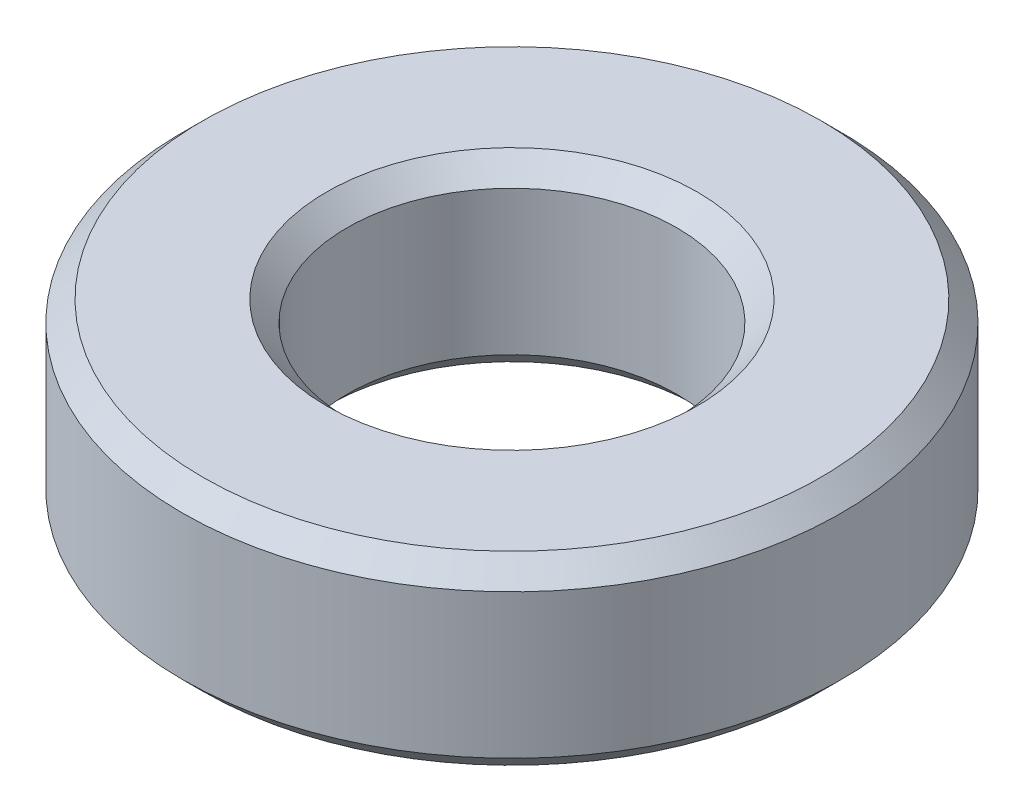
from build123d import *

# Parameters (mm, degrees)
SKETCH1_R           = 8
SKETCH1_R_2         = 4
BOSS_EXTRUDE1_DEPTH = 4.5
CHAMFER1_SIZE       = 0.5


with BuildPart() as part:
    # Sketch1 → Boss-Extrude1 (new body)
    with BuildSketch(Plane(origin=(0, 0, 0), x_dir=(1, 0, 0), z_dir=(0, 1, 0))):
        with Locations(Location((0, 0, 0), (0, 0, 270))):
            Circle(SKETCH1_R)
        with Locations(Location((0, 0, 0), (0, 0, 270))):
            Circle(SKETCH1_R_2, mode=Mode.SUBTRACT)
    extrude(amount=BOSS_EXTRUDE1_DEPTH)

    # Chamfer1
    chamfer1_edges = [part.edges().sort_by_distance(p)[0] for p in [
        (0, 0, -8),
        (0, 4.5, -8),
        (0, 0, -4),
        (0, 4.5, -4),
    ]]
    chamfer(chamfer1_edges, length=CHAMFER1_SIZE)


solid = part.part
